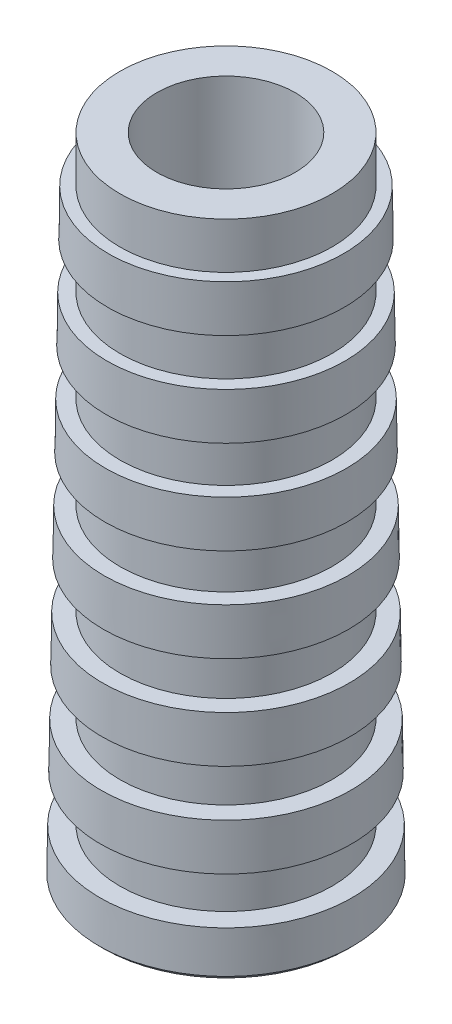
from build123d import *


with BuildPart() as part:
    # 草图1 → 旋转1 (revolve)
    with BuildSketch(Plane(origin=(0, 0, 0), x_dir=(-1, 0, 0), z_dir=(0, 0, -1)), mode=Mode.PRIVATE) as revolve_1_sk:
        Polygon((-23, -215), (-26.422241501, -215), (-26.576207001, -225), (-23, -225), (-23, -235), (-26.730172501, -235), (-26.884138001, -245), (-23, -245), (-23, -255), (-27.038103501, -255), (-27.192069, -265), (-23, -265), (-23, -275), (-27.3460345, -275), (-27.484836909, -284.015163091), (-26.5, -285), (-16, -285), (-15, -284), (-15, -145), (-23, -145), (-23, -155), (-25.498448502, -155), (-25.652414002, -165), (-23, -165), (-23, -175), (-25.806379502, -175), (-25.960345002, -185), (-23, -185), (-23, -195), (-26.114310502, -195), (-26.268276001, -205), (-23, -205), align=None)
    revolve(revolve_1_sk.sketch.rotate(Axis((0, -285, 0), (0, 1, 0)), 180), axis=Axis((0, -285, 0), (0, 1, 0)))


solid = part.part
